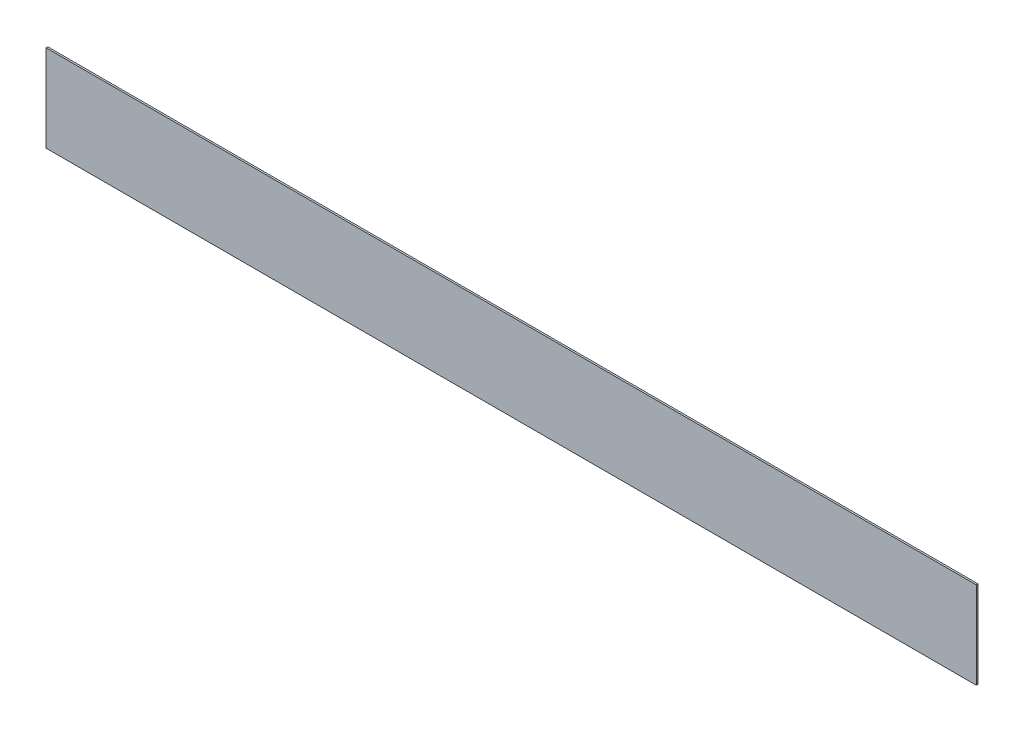
from build123d import *

# Parameters (mm, degrees)
SKETCH_1_W      = 2140
SKETCH_1_H      = 200
EXTRUDE_1_DEPTH = 4


with BuildPart() as part:
    # 草图1 → 凸台-拉伸1 (new body)
    with BuildSketch(Plane.XY):
        Rectangle(SKETCH_1_W, SKETCH_1_H)
    extrude(amount=EXTRUDE_1_DEPTH)


solid = part.part
